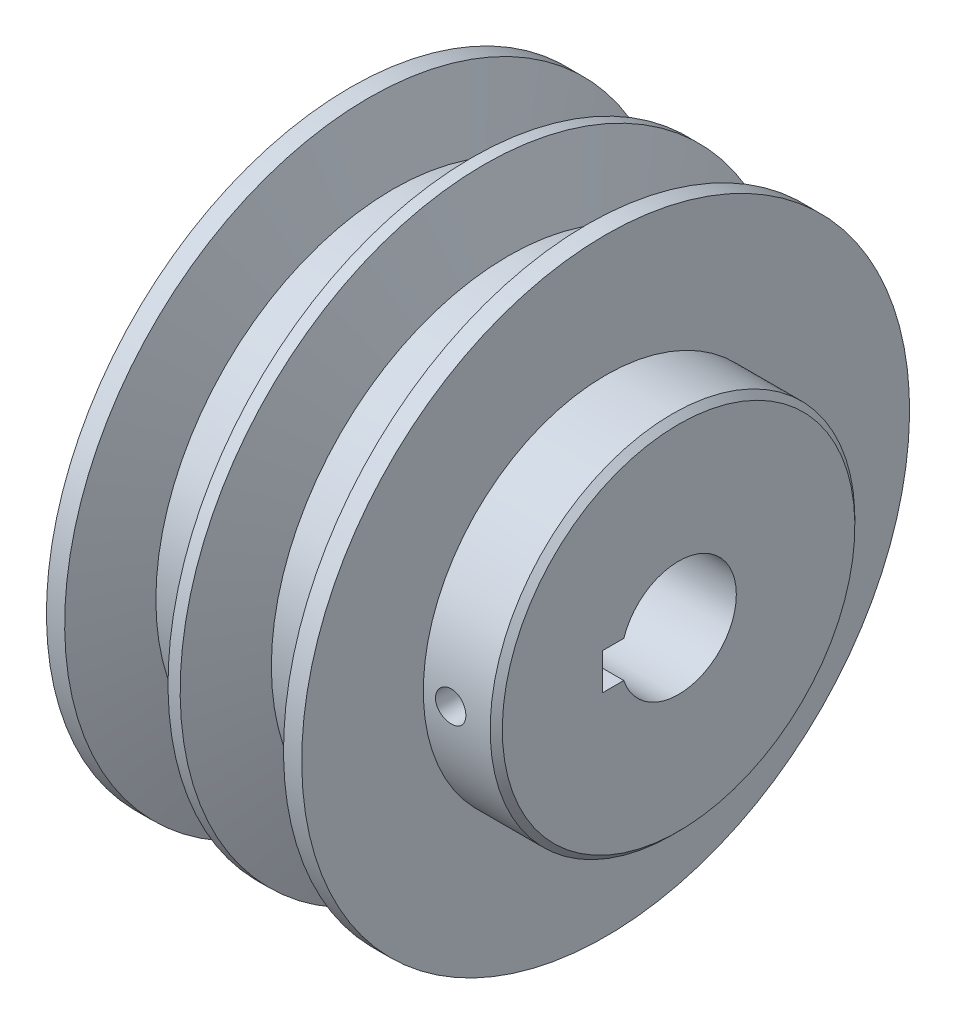
from build123d import *

# Parameters (mm, degrees)
SKETCH2_R          = 9.5
CUT_EXTRUDE1_DEPTH = 70
CHAMFER1_SIZE      = 1
SKETCH7_W          = 6
SKETCH7_H          = 6
CUT_EXTRUDE2_DEPTH = 70


with BuildPart() as part:
    # Sketch1 → Revolve1 (revolve)
    with BuildSketch(Plane.XY):
        Polygon((0, 0), (0, 50), (3, 50), (7.003672577, 39), (15.996327423, 39), (20, 50), (22, 50), (26.003672577, 39), (34.996327423, 39), (39, 50), (42, 50), (42, 30), (54, 30), (54, 0), align=None)
    revolve(axis=Axis((54, 0, 0), (-1, 0, 0)))

    # Sketch2 → Cut-Extrude1 (cut)
    with BuildSketch(Plane(origin=(54, 0, 0), x_dir=(0, 0, -1), z_dir=(1, 0, 0))):
        with Locations(Location((0, 0, 0), (0, 0, 90))):
            Circle(SKETCH2_R)
    extrude(amount=-CUT_EXTRUDE1_DEPTH, mode=Mode.SUBTRACT)

    # Sketch5 → M6 Tapped Hole1 (revolve, cut)
    with BuildSketch(Plane.YZ.offset(46.5)):
        Polygon((0, 0), (0, 51.502151548), (2.5, 50), (2.5, 0), align=None)
    revolve(axis=Axis((46.5, 0, -6.35), (0, 0, 1)), mode=Mode.SUBTRACT)

    # Chamfer1
    chamfer1_edges = [part.edges().sort_by_distance(p)[0] for p in [
        (54, -30, 0),
    ]]
    chamfer(chamfer1_edges, length=CHAMFER1_SIZE)

    # Sketch7 → Cut-Extrude2 (cut)
    with BuildSketch(Plane(origin=(54, 0, 0), x_dir=(0, 0, -1), z_dir=(1, 0, 0))):
        with Locations((-9.5, 0)):
            Rectangle(SKETCH7_W, SKETCH7_H)
    extrude(amount=-CUT_EXTRUDE2_DEPTH, mode=Mode.SUBTRACT)


solid = part.part
